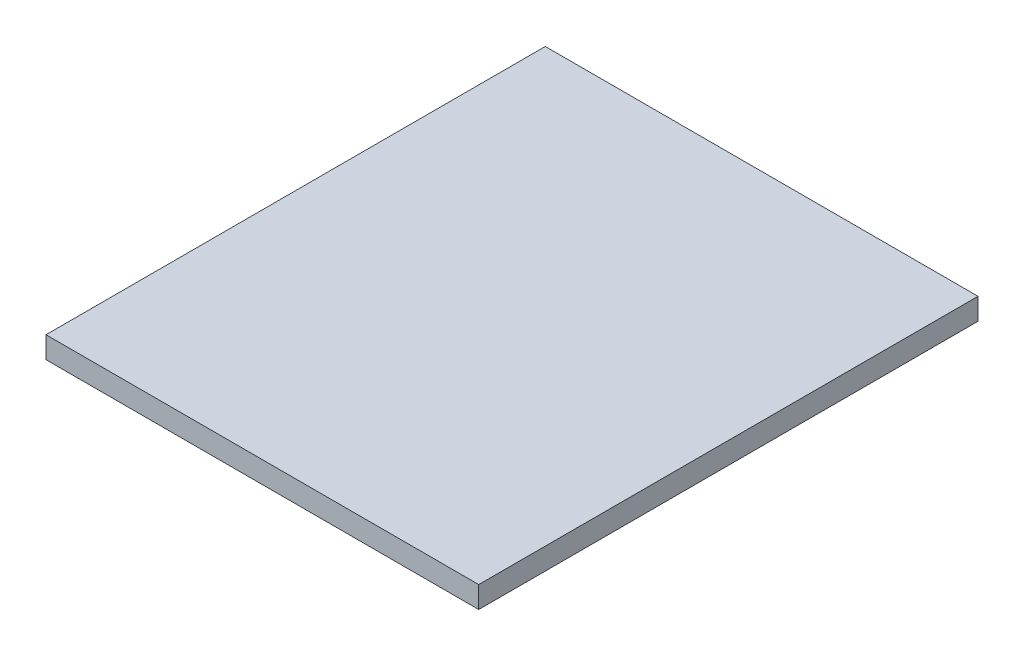
from build123d import *

# Parameters (mm, degrees)
SKETCH1_W           = 130
SKETCH1_H           = 150
BOSS_EXTRUDE1_DEPTH = 6.5


with BuildPart() as part:
    # Sketch1 → Boss-Extrude1 (new body)
    with BuildSketch(Plane(origin=(0, 0, 0), x_dir=(1, 0, 0), z_dir=(0, 1, 0))):
        Rectangle(SKETCH1_W, SKETCH1_H)
    extrude(amount=BOSS_EXTRUDE1_DEPTH)


solid = part.part
